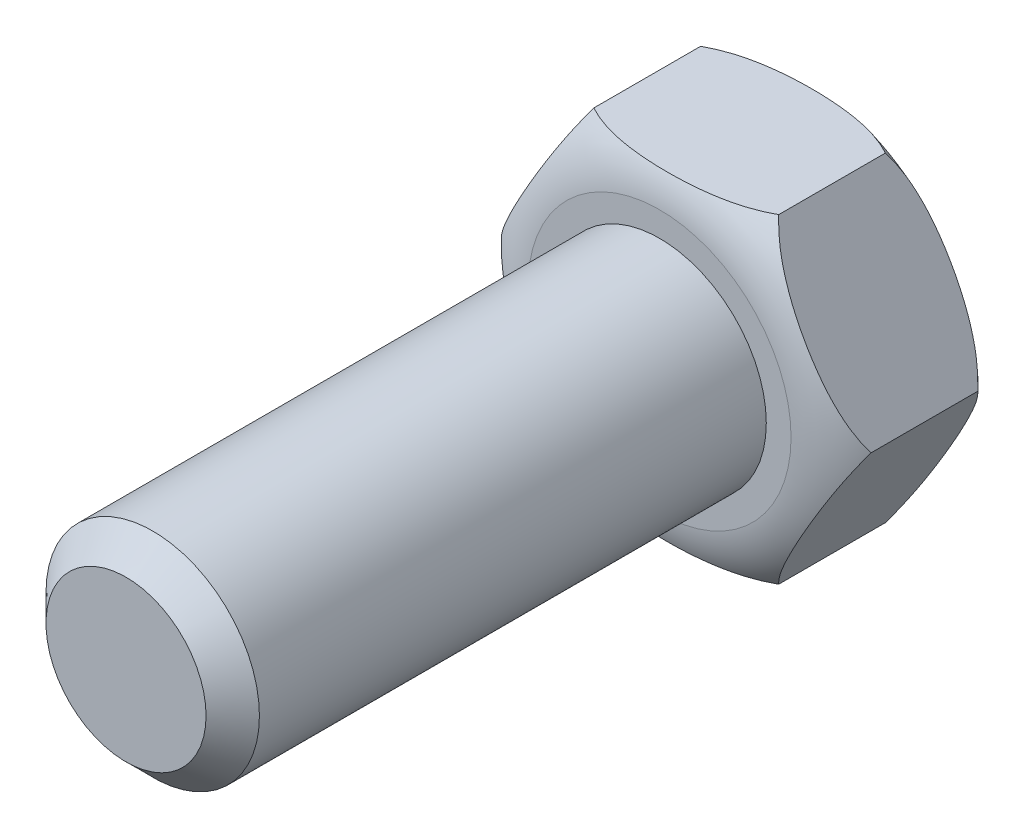
from build123d import *

# Parameters (mm, degrees)
BOSS_EXTRUDE1_DEPTH = 6
SKETCH2_R           = 4
BOSS_EXTRUDE2_DEPTH = 20
CHAMFER1_SIZE       = 1
SCALE_1_SCALE       = 1.875


with BuildPart() as part:
    # Sketch1 → Boss-Extrude1 (new body)
    with BuildSketch(Plane.XY):
        Polygon((6.92820323, 0), (3.464101615, 6), (-3.464101615, 6), (-6.92820323, 0), (-3.464101615, -6), (3.464101615, -6), align=None)
    extrude(amount=BOSS_EXTRUDE1_DEPTH)

    # Sketch2 → Boss-Extrude2 (add)
    with BuildSketch(Plane.XY.offset(6)):
        Circle(SKETCH2_R)
    extrude(amount=BOSS_EXTRUDE2_DEPTH)

    # Chamfer1
    chamfer1_edges = [part.edges().sort_by_distance(p)[0] for p in [
        (-4, 0, 26),
    ]]
    chamfer(chamfer1_edges, length=CHAMFER1_SIZE)

    # Sketch3 → Cut-Revolve1 (revolve, cut)
    with BuildSketch(Plane(origin=(0, 0, 0), x_dir=(1, 0, 0), z_dir=(0, 1, 0)), mode=Mode.PRIVATE) as cut_revolve1_sk:
        with BuildLine():
            ThreePointArc((-6.92820323, -1), (-6.024854057, -0.306698347), (-4.92820323, 0))
            Line((-4.92820323, 0), (-8.853828921, 0.851275599))
            Line((-8.853828921, 0.851275599), (-9.311272628, -1))
            Line((-9.311272628, -1), (-6.92820323, -1))
        make_face()
        with BuildLine():
            ThreePointArc((-6.92820323, -5), (-6.024854057, -5.693301653), (-4.92820323, -6))
            Line((-4.92820323, -6), (-8.016018434, -6.744872817))
            Line((-8.016018434, -6.744872817), (-9.311272628, -5))
            Line((-9.311272628, -5), (-6.92820323, -5))
        make_face()
    revolve(cut_revolve1_sk.sketch.rotate(Axis((0, 0, 0), (0, 0, -1)), 180), axis=Axis((0, 0, 0), (0, 0, -1)), mode=Mode.SUBTRACT)


with BuildPart() as part_1:
    # Scale 1: scaled about (1e-08, -1e-08, 10.434688187)
    add(part.part.scale(SCALE_1_SCALE).moved(Location((-9e-09, 9e-09, -9.130352164))))


solid = part_1.part
